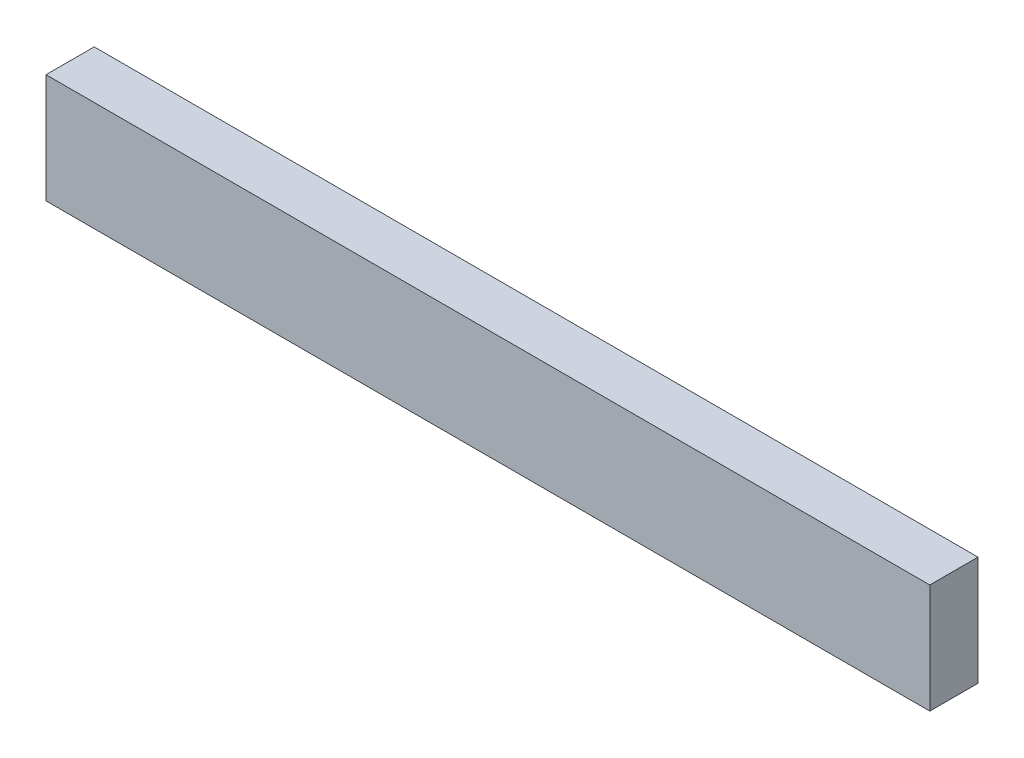
SolidWorks part; units mm, degrees
ref_plane "前视基准面" through (0, 0, 0) normal (0, 0, 1) x (1, 0, 0)
ref_plane "上视基准面" through (0, 0, 0) normal (0, 1, 0) x (1, 0, 0)
ref_plane "右视基准面" through (0, 0, 0) normal (1, 0, 0) x (0, 0, -1)
sketch "草图1" plane through (0, 0, 0) normal (0, 0, 1) x (1, 0, 0)
  line L1 (-137.5, -17) -> (137.5, -17)
  line L2 (-137.5, -17) -> (-137.5, 17)
  line L3 (-137.5, 17) -> (137.5, 17)
  line L4 (137.5, -17) -> (137.5, 17)
  line L5 (-137.5, -17) -> (137.5, 17) construction
  line L6 (-137.5, 17) -> (137.5, -17) construction
  point P0 (0, 0)
  dimension "D1" = 275
  dimension "D2" = 34
extrude "凸台-拉伸1" add sketch "草图1" along normal blind 15
